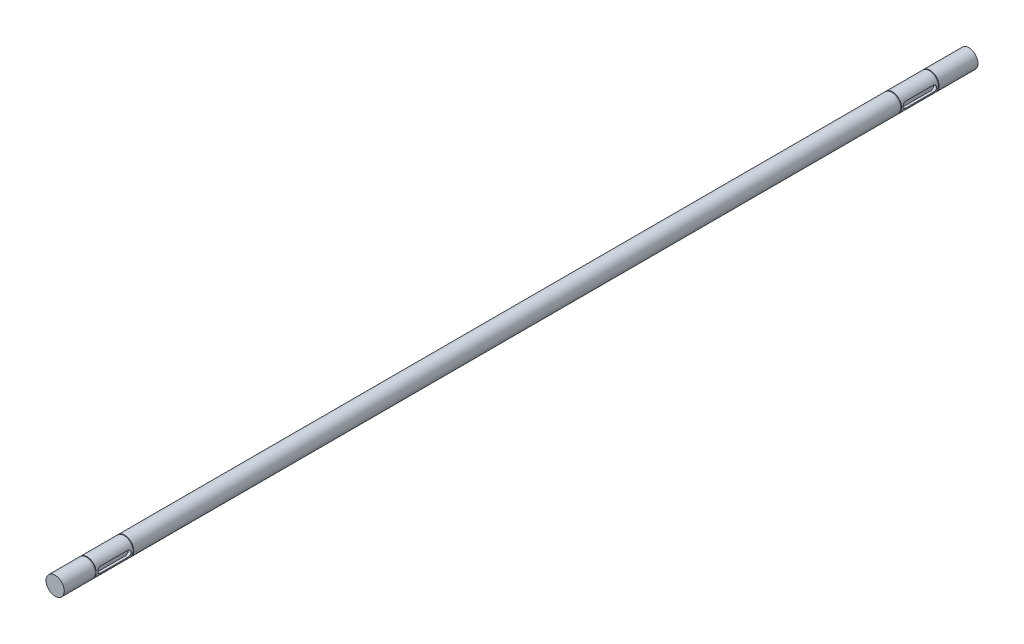
from build123d import *

# Parameters (mm, degrees)
SKETCH_2_R             = 15
EXTRUDE_1_DEPTH        = 1500
CUT_EXTRUDE_1_DEPTH    = 1501.283306579
SKETCH_4_W             = 1.6
SKETCH_4_H             = 0.7
PATTERN_LINEAR_1_COUNT = 2
PATTERN_LINEAR_1_PITCH = 1322
HOLE_WIZARD_M8_1_D     = 6.8
HOLE_WIZARD_M8_1_DEPTH = 19.75
HOLE_WIZARD_M8_1_TIP   = 2.042926105


with BuildPart() as part:
    # 草图2 → 凸台-拉伸1 (new body)
    with BuildSketch(Plane.XY):
        Circle(SKETCH_2_R)
    extrude(amount=EXTRUDE_1_DEPTH)

    # 草图3 → 切除-拉伸1 (cut, through all)
    with BuildSketch(Plane(origin=(10, 0, 0), x_dir=(0, 0, -1), z_dir=(1, 0, 0))):
        with BuildLine():
            Line((-1440, 5), (-1395, 5))
            ThreePointArc((-1395, 5), (-1390, 0), (-1395, -5))
            Line((-1395, -5), (-1440, -5))
            ThreePointArc((-1440, -5), (-1445, 0), (-1440, 5))
        make_face()
        with BuildLine():
            Line((-73, -5), (-118, -5))
            ThreePointArc((-118, -5), (-123, 0), (-118, 5))
            Line((-118, 5), (-73, 5))
            ThreePointArc((-73, 5), (-68, 0), (-73, -5))
        make_face()
    extrude(amount=CUT_EXTRUDE_1_DEPTH, mode=Mode.SUBTRACT)

    # 草图4 → 切除-旋转5 (revolve, cut)
    with BuildSketch(Plane(origin=(0, 0, 0), x_dir=(0, 0, -1), z_dir=(1, 0, 0))):
        with Locations((-1448.3, 14.65)):
            Rectangle(SKETCH_4_W, SKETCH_4_H)
        with Locations((-1386.7, 14.65)):
            Rectangle(SKETCH_4_W, SKETCH_4_H)
    cut_revolve_5 = revolve(axis=Axis((0, 0, 1445), (0, 0, 1)), mode=Mode.SUBTRACT)

    # 阵列(线性)1: 切除-旋转5 ×2
    with Locations(*[(0, 0, -i * PATTERN_LINEAR_1_PITCH) for i in range(1, PATTERN_LINEAR_1_COUNT)]):
        add(cut_revolve_5, mode=Mode.SUBTRACT)

    # M8 螺纹孔1
    with Locations(Plane(origin=(0, 0, 0), x_dir=(-1, 0, 0), z_dir=(0, 0, -1))):
        with Locations((0, 0)):
            Hole(HOLE_WIZARD_M8_1_D / 2, depth=HOLE_WIZARD_M8_1_DEPTH)
            with Locations((0, 0, -(HOLE_WIZARD_M8_1_DEPTH + HOLE_WIZARD_M8_1_TIP / 2))):  # 118° drill point
                Cone(0, HOLE_WIZARD_M8_1_D / 2, HOLE_WIZARD_M8_1_TIP, mode=Mode.SUBTRACT)


solid = part.part
